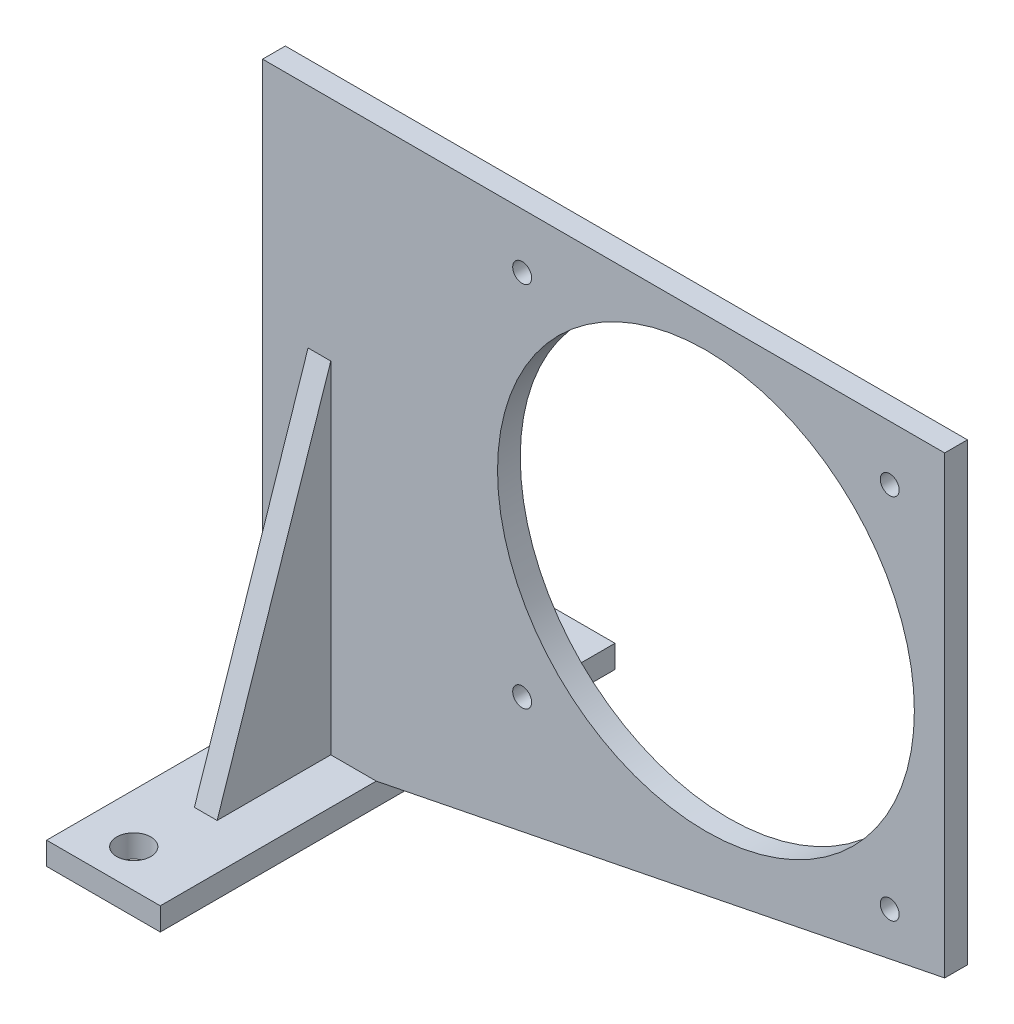
SolidWorks part; units mm, degrees
ref_plane "前视基准面" through (0, 0, 0) normal (0, 0, 1) x (1, 0, 0)
ref_plane "上视基准面" through (0, 0, 0) normal (0, 1, 0) x (1, 0, 0)
ref_plane "右视基准面" through (0, 0, 0) normal (1, 0, 0) x (0, 0, -1)
sketch "草图1" plane through (0, 0, 0) normal (0, 0, 1) x (1, 0, 0)
  line L0 (68.5, 87) -> (165.5, 87) construction
  line L1 (0, 0) -> (30, 0)
  line L2 (0, 0) -> (0, 150)
  line L3 (0, 150) -> (180, 150)
  line L4 (180, 30) -> (180, 150)
  line L5 (117, 38.5) -> (117, 165.507) construction
  line L6 (68.5, 135.5) -> (165.5, 135.5) construction
  line L7 (68.5, 135.5) -> (68.5, 38.5) construction
  line L8 (68.5, 38.5) -> (165.5, 38.5) construction
  line L9 (165.5, 135.5) -> (165.5, 38.5) construction
  line L10 (180, 30) -> (30, 0)
  circle A0 centre (165.5, 135.5) radius 2.5
  circle A1 centre (68.5, 135.5) radius 2.5
  circle A2 centre (165.5, 38.5) radius 2.5
  circle A3 centre (68.5, 38.5) radius 2.5
  circle A4 centre (117, 87) radius 55
  dimension "D7" = 5
  dimension "D8" = 5
  dimension "D9" = 5
  dimension "D10" = 5
  dimension "D11" = 30
  dimension "D5" = 110
  dimension "D2" = 120
  dimension "D3" = 97
  dimension "D4" = 97
  dimension "D6" = 63
  dimension "D12" = 63
  dimension "D13" = 30
  dimension "D14" = 180
extrude "凸台-拉伸1" add sketch "草图1" along normal blind 6
sketch "草图4" plane through (0, 0, 0) normal (0, -1, 0) x (1, 0, 0)
  line L0 (30, 6) -> (30, 0) construction
  line L1 (0, 63) -> (30, 63)
  line L2 (0, 63) -> (0, -57)
  line L3 (0, -57) -> (30, -57)
  line L4 (30, 63) -> (30, -57)
  line L5 (0, 6) -> (0, 0) construction
  line L6 (180, 3) -> (-18.2918, 3) construction
  line L7 (180, 6) -> (180, 0) construction
  dimension "D1" = 120
  dimension "D2" = 60
extrude "凸台-拉伸3" add sketch "草图4" along normal blind 6
sketch "草图5" plane through (0, 0, 0) normal (0, 1, 0) x (1, 0, 0)
  line L0 (13, 65.9001) -> (13, -75.7547) construction
  line L1 (0, 0) -> (0, 57) construction
  line L2 (180, -3) -> (-15.5184, -3) construction
  line L3 (180, -6) -> (180, 0) construction
  circle A0 centre (13, 47) radius 4.5
  circle A1 centre (13, -53) radius 4.5
  dimension "D2" = 9
  dimension "D3" = 9
  dimension "D4" = 100
  dimension "D5" = 50
  dimension "D1" = 13
extrude "切除-拉伸1" cut sketch "草图5" against normal blind 6
ref_plane "基准面1" through (15, 0, 0) normal (-1, 0, 0) x (0, 0, 1)
sketch "草图6" plane through (15, 0, 0) normal (-1, 0, 0) x (0, 0, 1)
  line L0 (0, 90) -> (-30, 0)
  line L1 (0, 150) -> (0, 0) construction
  line L2 (0, 0) -> (-57, 0) construction
  line L3 (-30, 0) -> (0, 0)
  line L4 (0, 0) -> (0, 90)
  line L5 (3, 150) -> (3, -25.7011) construction
  line L6 (6, 150) -> (0, 150) construction
  line L7 (6, 0) -> (6, 90)
  line L8 (36, 0) -> (6, 0)
  line L9 (6, 90) -> (36, 0)
  dimension "D1" = 30
  dimension "D2" = 90
extrude "凸台-拉伸4" add sketch "草图6" along normal blind 3 and the other way blind 3
